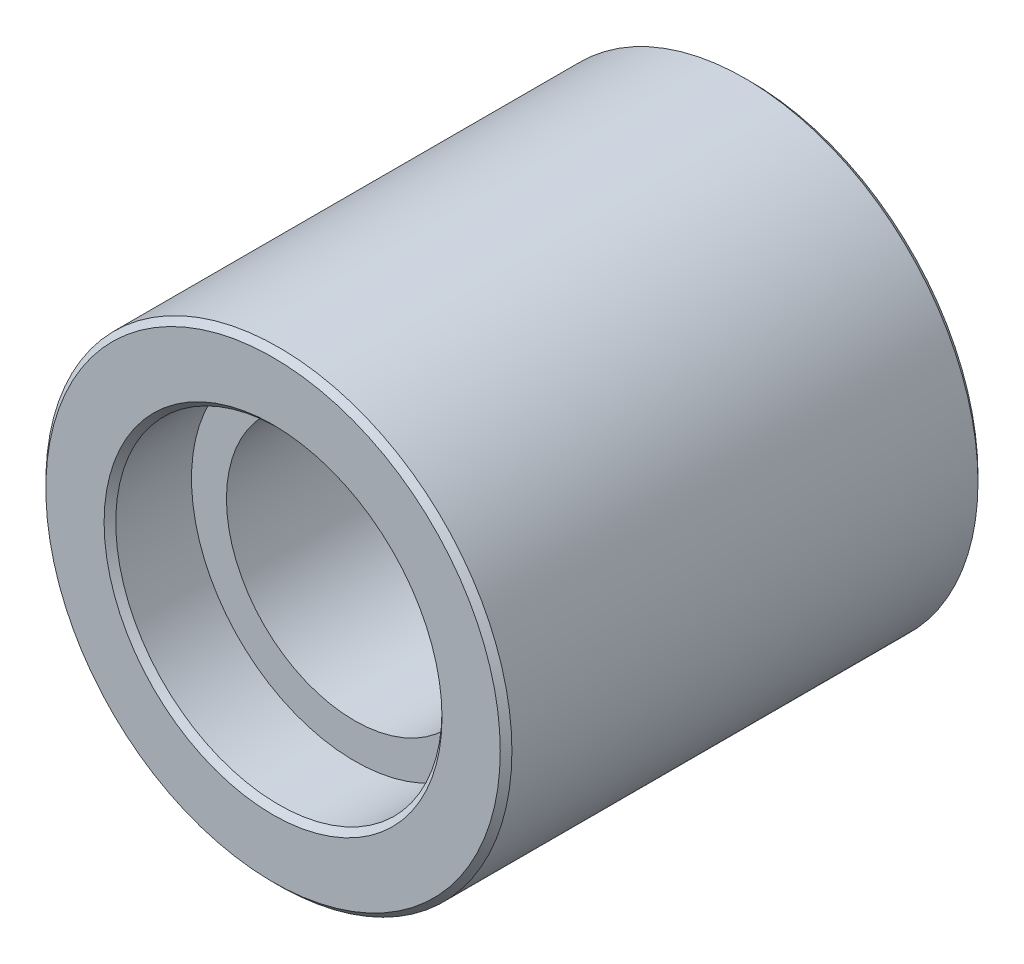
from build123d import *

# Parameters (mm, degrees)
SKETCH_2_R          = 20
SKETCH_2_R_2        = 11
EXTRUDE_1_DEPTH     = 20.5
SKETCH_3_R          = 14
CUT_EXTRUDE_1_DEPTH = 7
CHAMFER_3_SIZE      = 0.5


with BuildPart() as part:
    # 草图2 → 凸台-拉伸1 (new, symmetric)
    with BuildSketch(Plane.XY):
        Circle(SKETCH_2_R)
        Circle(SKETCH_2_R_2, mode=Mode.SUBTRACT)
    extrude(amount=EXTRUDE_1_DEPTH, both=True)

    # 草图3 → 切除-拉伸1 (cut)
    with BuildSketch(Plane.XY.offset(20.5)):
        Circle(SKETCH_3_R)
    cut_extrude_1 = extrude(amount=-CUT_EXTRUDE_1_DEPTH, mode=Mode.SUBTRACT)

    # 镜向6: 切除-拉伸1 across plane
    add(cut_extrude_1.mirror(Plane.XY), mode=Mode.SUBTRACT)

    # 倒角3
    chamfer_3_edges = [part.edges().sort_by_distance(p)[0] for p in [
        (-14, 0, 20.5),
        (-14, 0, -20.5),
        (-20, 0, -20.5),
        (-20, 0, 20.5),
    ]]
    chamfer(chamfer_3_edges, length=CHAMFER_3_SIZE)


solid = part.part
